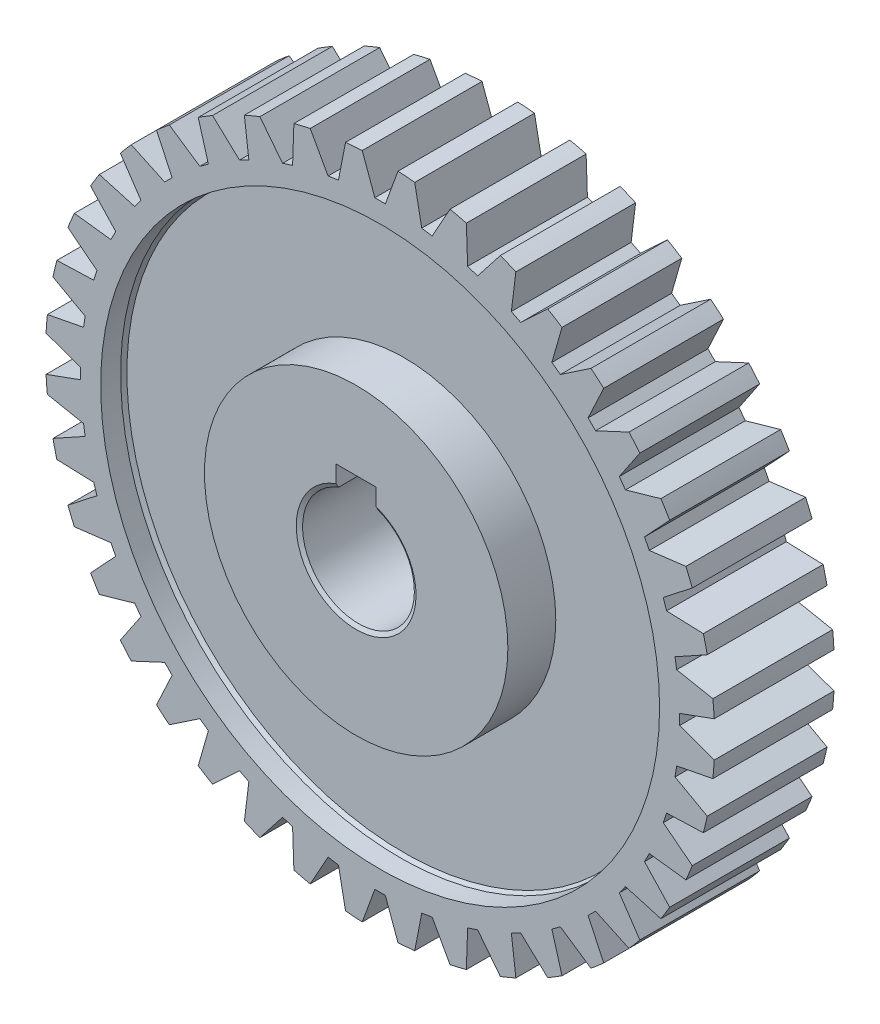
from build123d import *
from OCP.BRepFilletAPI import BRepFilletAPI_MakeChamfer

# Parameters (mm, degrees)
SKETCH1_R           = 41.895
BOSS_EXTRUDE1_DEPTH = 15
SKETCH2_R           = 12
BOSS_EXTRUDE2_DEPTH = 3
SKETCH3_R           = 35
SKETCH3_R_2         = 19
CUT_EXTRUDE1_DEPTH  = 3
BOSS_EXTRUDE3_START = 3
SKETCH4_R           = 19
BOSS_EXTRUDE3_DEPTH = 3
CUT_EXTRUDE2_DEPTH  = 63.860019488
CUT_EXTRUDE3_DEPTH  = 26
CIRPATTERN1_COUNT   = 40
CHAMFER1_SIZE       = 0.5
CHAMFER1_SIZE2      = 0.288675135
CHAMFER2_SIZE       = 0.5
CHAMFER2_SIZE2      = 0.288675135


with BuildPart() as part:
    # Sketch1 → Boss-Extrude1 (new body)
    with BuildSketch(Plane.XY):
        Circle(SKETCH1_R)
    extrude(amount=BOSS_EXTRUDE1_DEPTH)

    # Sketch2 → Boss-Extrude2 (add)
    with BuildSketch(Plane(origin=(0, 0, 0), x_dir=(-1, 0, 0), z_dir=(0, 0, -1))):
        Circle(SKETCH2_R)
    extrude(amount=BOSS_EXTRUDE2_DEPTH)

    # Sketch3 → Cut-Extrude1 (cut)
    with BuildSketch(Plane.XY.offset(15)):
        Circle(SKETCH3_R)
        Circle(SKETCH3_R_2, mode=Mode.SUBTRACT)
    extrude(amount=-CUT_EXTRUDE1_DEPTH, mode=Mode.SUBTRACT)

    # Sketch4 → Boss-Extrude3 (add)
    with BuildSketch(Plane.XY.offset(15).offset(BOSS_EXTRUDE3_START)):
        Circle(SKETCH4_R)
    extrude(amount=-BOSS_EXTRUDE3_DEPTH)

    # Sketch5 → Cut-Extrude2 (cut, through all)
    with BuildSketch(Plane.XY.offset(18)):
        with BuildLine():
            Line((2.5, 9.2), (-2.5, 9.2))
            Line((-2.5, 9.2), (-2.5, 6.538348415))
            ThreePointArc((-2.5, 6.538348415), (0, 7), (2.5, 6.538348415))
            Line((2.5, 6.538348415), (2.5, 9.2))
        make_face()
        with BuildLine():
            ThreePointArc((2.5, 6.538348415), (0, 7), (-2.5, 6.538348415))
            Line((-2.5, 6.538348415), (-2.5, 4.8))
            Line((-2.5, 4.8), (2.5, 4.8))
            Line((2.5, 4.8), (2.5, 6.538348415))
        make_face()
        with BuildLine():
            Line((-2.5, 4.8), (-2.5, 6.538348415))
            ThreePointArc((-2.5, 6.538348415), (-3.968626967, -5.766281297), (7, 0))
            ThreePointArc((7, 0), (5.766281297, 3.968626967), (2.5, 6.538348415))
            Line((2.5, 6.538348415), (2.5, 4.8))
            Line((2.5, 4.8), (-2.5, 4.8))
        make_face()
    extrude(amount=-CUT_EXTRUDE2_DEPTH, mode=Mode.SUBTRACT)

    # Sketch6 → Cut-Extrude3 (cut)
    with BuildSketch(Plane.XY):
        Polygon((0.660074414, 37.5), (-0.660074414, 37.5), (-3.23503061, 44.574634003), (3.23503061, 44.574634003), align=None)
    cut_extrude3 = extrude(amount=CUT_EXTRUDE3_DEPTH, mode=Mode.SUBTRACT)

    # CirPattern1: Cut-Extrude3 ×40 about axis
    cirpattern1_axis = Axis((0, 0, 0), (0, 0, 1))
    for i in range(1, CIRPATTERN1_COUNT):
        add(cut_extrude3.rotate(cirpattern1_axis, i * 360 / CIRPATTERN1_COUNT), mode=Mode.SUBTRACT)

    # Chamfer1: one chamfer whose edges measure the first distance from different faces: ONE call of the kernel's chamfer builder (chamfer() names one face for all edges)
    chamfer1_edges_1 = [part.edges().sort_by_distance(p)[0] for p in [
        (-3.968626967, -5.766281297, -3),
    ]]
    chamfer1_side_1 = [part.faces().sort_by_distance(p)[0] for p in [
        (-3.968626967, -5.766281297, 7.5),
    ]]
    chamfer1_edges_2 = [part.edges().sort_by_distance(p)[0] for p in [
        (-3.968626967, -5.766281297, 18),
    ]]
    chamfer1_side_2 = [part.faces().sort_by_distance(p)[0] for p in [
        (-18.462598846, 0, 18),
    ]]
    chamfer1 = BRepFilletAPI_MakeChamfer(part.part.solid().wrapped)
    for e in chamfer1_edges_1:
        chamfer1.Add(CHAMFER1_SIZE, CHAMFER1_SIZE2, e.wrapped, chamfer1_side_1[0].wrapped)  # the first distance lies on this face
    for e in chamfer1_edges_2:
        chamfer1.Add(CHAMFER1_SIZE, CHAMFER1_SIZE2, e.wrapped, chamfer1_side_2[0].wrapped)  # the first distance lies on this face
    add(Compound.cast(chamfer1.Shape()), mode=Mode.REPLACE)

    # Chamfer2
    chamfer2_edges = [part.edges().sort_by_distance(p)[0] for p in [
        (-35, 0, 12),
    ]]
    chamfer2_side = [part.faces().sort_by_distance(p)[0] for p in [
        (-35, 0, 13.5),
    ]]
    chamfer(chamfer2_edges, length=CHAMFER2_SIZE, length2=CHAMFER2_SIZE2, reference=chamfer2_side[0])


solid = part.part
